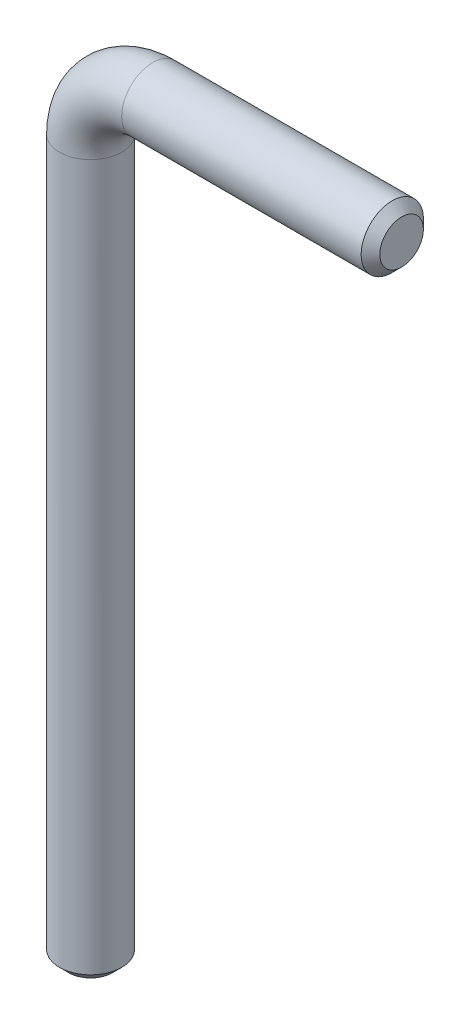
SolidWorks part; units mm, degrees
ref_plane "前视基准面" through (0, 0, 0) normal (0, 0, 1) x (1, 0, 0)
ref_plane "上视基准面" through (0, 0, 0) normal (0, 1, 0) x (1, 0, 0)
ref_plane "右视基准面" through (0, 0, 0) normal (1, 0, 0) x (0, 0, -1)
sketch "草图1" plane through (0, 0, 0) normal (0, 0, 1) x (1, 0, 0)
  line L0 (0, -20) -> (0, -250)
  line L1 (20, 0) -> (100, 0)
  arc A0 (20, 0) -> (0, -20) centre (20, -20) ccw
  point P6 (0, 0)
  dimension "D3" = 20
  dimension "D1" = 250
  dimension "D2" = 100
sweep "扫描1" add path "草图1" circular profile diameter 20 parameters "D3"=20
chamfer "倒角1" distance 3 angle 45 1 edges at (0, -250, 10)
chamfer "倒角2" distance 3 angle 45 1 edges at (100, 0, 10)
